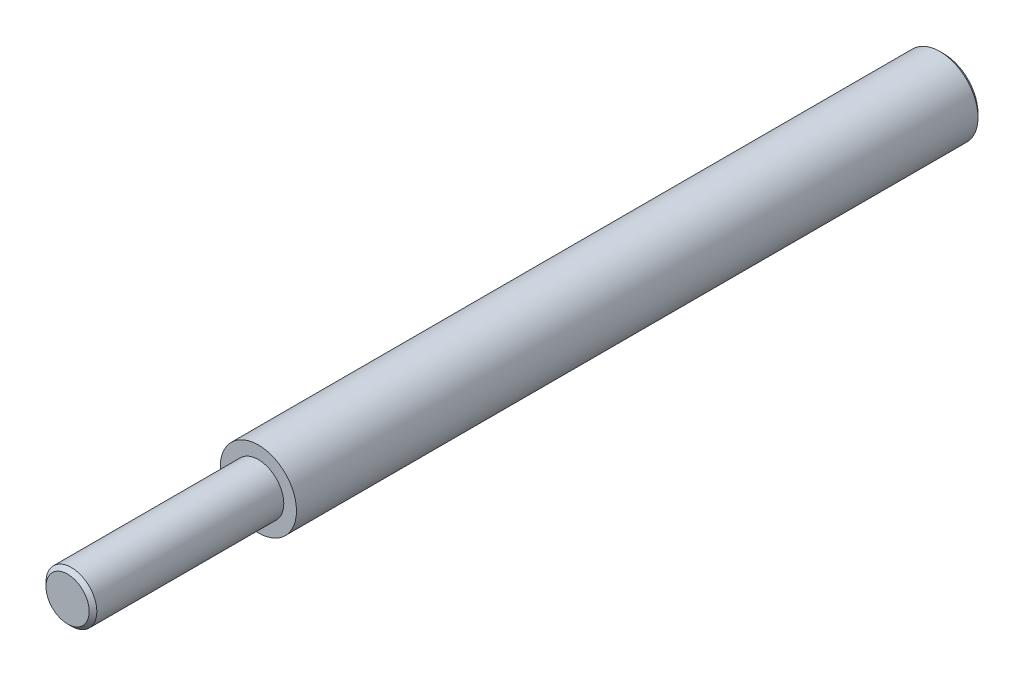
from build123d import *

# Parameters (mm, degrees)
SKETCH1_R           = 5.4
BOSS_EXTRUDE1_DEPTH = 124
CUT_EXTRUDE1_START  = -27
SKETCH2_R           = 5.4
SKETCH2_R_2         = 3.6
CUT_EXTRUDE1_DEPTH  = 27
CHAMFER1_SIZE       = 0.54


with BuildPart() as part:
    # Sketch1 → Boss-Extrude1 (new body)
    with BuildSketch(Plane.XY):
        Circle(SKETCH1_R)
    extrude(amount=BOSS_EXTRUDE1_DEPTH)

    # Sketch2 → Cut-Extrude1 (cut)
    with BuildSketch(Plane.XY.offset(124).offset(CUT_EXTRUDE1_START)):
        Circle(SKETCH2_R)
        Circle(SKETCH2_R_2, mode=Mode.SUBTRACT)
    extrude(amount=CUT_EXTRUDE1_DEPTH, mode=Mode.SUBTRACT)

    # Chamfer1
    chamfer1_edges = [part.edges().sort_by_distance(p)[0] for p in [
        (-5.4, 0, 0),
        (-3.6, 0, 124),
    ]]
    chamfer(chamfer1_edges, length=CHAMFER1_SIZE)


solid = part.part
